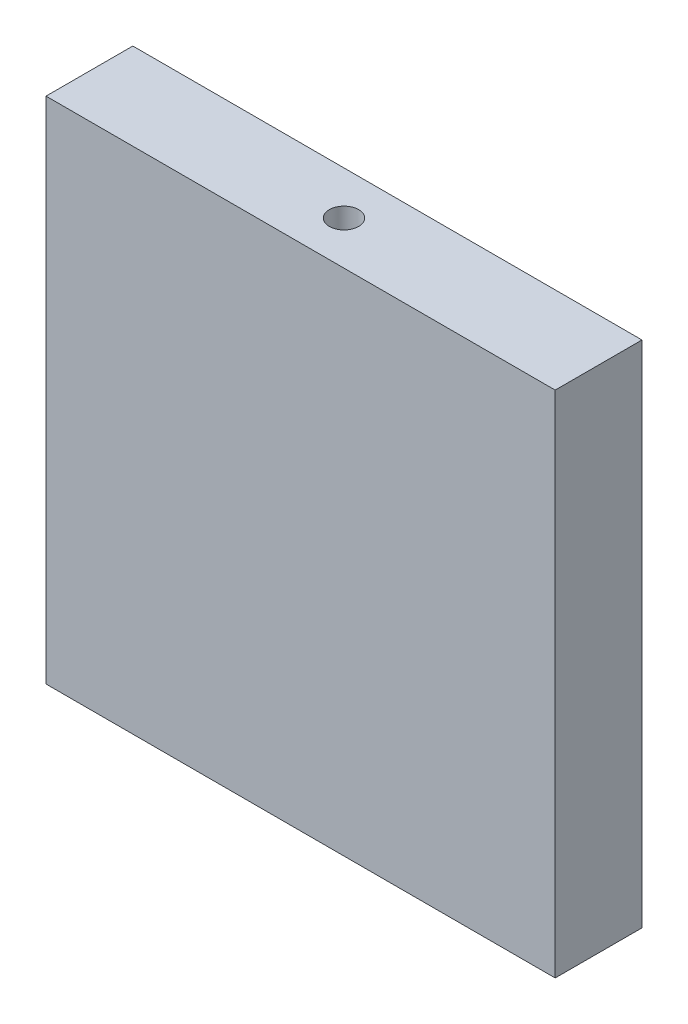
SolidWorks part; units mm, degrees
ref_plane "Front Plane" through (0, 0, 0) normal (0, 0, 1) x (1, 0, 0)
ref_plane "Top Plane" through (0, 0, 0) normal (0, 1, 0) x (1, 0, 0)
ref_plane "Right Plane" through (0, 0, 0) normal (1, 0, 0) x (0, 0, -1)
sketch "Sketch1" plane through (0, 0, 0) normal (0, 0, 1) x (1, 0, 0)
  line L1 (88, 88) -> (-88, 88)
  line L2 (88, 88) -> (88, -88)
  line L3 (88, -88) -> (-88, -88)
  line L4 (-88, 88) -> (-88, -88)
  line L5 (88, 88) -> (-88, -88) construction
  line L6 (88, -88) -> (-88, 88) construction
  point P0 (0, 0)
  dimension "D1" = 176
  dimension "D2" = 176
extrude "Boss-Extrude1" add sketch "Sketch1" along normal blind 30
sketch "Sketch3" plane through (0, 88, 0) normal (0, 1, 0) x (1, 0, 0)
  line L0 (-88, -30) -> (-88, 0) construction
  circle A0 centre (0, -15) radius 5.055
  point P4 (-88, -15)
  dimension "D1" = 10.11
extrude "Cut-Extrude1" cut sketch "Sketch3" against normal through all
